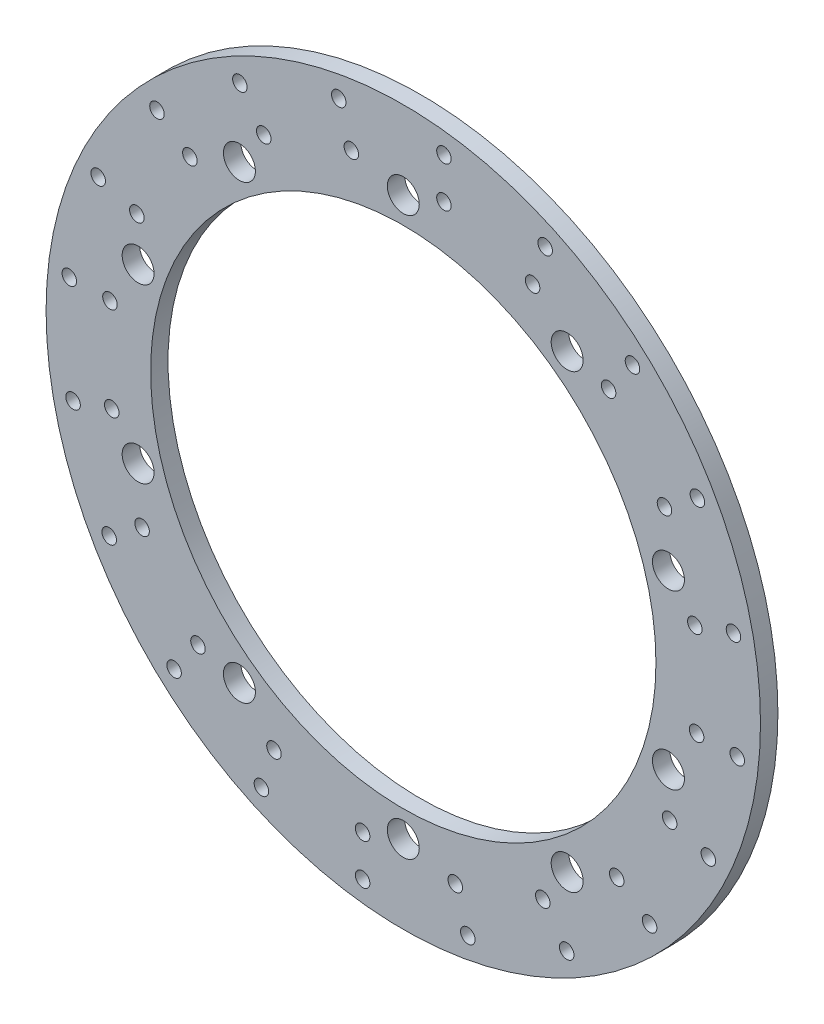
SolidWorks part; units mm, degrees
material "AL6061"
ref_plane "前视基准面" through (0, 0, 0) normal (0, 0, 1) x (1, 0, 0)
ref_plane "上视基准面" through (0, 0, 0) normal (0, 1, 0) x (1, 0, 0)
ref_plane "右视基准面" through (0, 0, 0) normal (1, 0, 0) x (0, 0, -1)
sketch "草图1" plane through (0, 0, 0) normal (0, 0, 1) x (1, 0, 0)
  circle A0 centre (0, 0) radius 61.5
  circle A1 centre (0, 0) radius 43.5
  dimension "D1" = 123
  dimension "D2" = 87
extrude "凸台-拉伸1" add sketch "草图1" along normal mid plane 3
hole_wizard "Ø5.5 (5.5) 直径孔2" positions "草图2" profile "草图3" hole size "Ø5.5" standard "GB" end condition through all
sketch "草图2" plane through (0, 0, 1.5) normal (0, 0, 1) x (1, 0, 0)
  line L0 (0, 45.7157) -> (0, -47.7003) construction
  circle A0 centre (0, 0) radius 48 construction
  point P0 (0, 48)
  dimension "D1" = 96
sketch "草图3" plane through (0, 48, 1.5) normal (1, 0, 0) x (0, -1, 0)
  line L0 (0, 0) -> (0, 3)
  line L1 (0, 3) -> (2.75, 3)
  line L2 (2.75, 3) -> (2.75, 0)
  line L5 (2.75, 0) -> (0, 0)
  line L11 (0, -6.35) -> (0, 107.95) construction
  dimension "通孔孔直径" = 5.5
  dimension "通孔孔深度" = 3
hole_wizard "M3 螺纹孔1" positions "草图4" profile "草图5" tap size "M3" standard "GB" end condition through all
sketch "草图4" plane through (0, 0, 1.5) normal (0, 0, 1) x (1, 0, 0)
  line L0 (-54, 9.4408) -> (-54, -2.1263) construction
  line L1 (5.6135, 0) -> (-69.2327, 0) construction
  point P0 (-57.5, 7)
  point P2 (-50.5, 7)
  dimension "D1" = 54
  dimension "D2" = 7
  dimension "D3" = 7
sketch "草图5" plane through (-57.5, 7, 1.5) normal (1, 0, 0) x (0, -1, 0)
  line L0 (0, 0) -> (0, 3)
  line L1 (0, 3) -> (1.25, 3)
  line L2 (1.25, 3) -> (1.25, 0)
  line L5 (1.25, 0) -> (0, 0)
  line L11 (0, -6.35) -> (0, 107.95) construction
  dimension "通孔螺纹孔钻头直径" = 2.5
  dimension "通孔螺纹孔钻头深度" = 3
cosmetic thread "孔螺蚊线1" parameters "D2"=3
cosmetic thread "孔螺蚊线2" parameters "D2"=3
pattern_circular "阵列(圆周)1" count 10 over 360 about axis through (0, 0, 0) along (0, 0, 1) of "Ø5.5 (5.5) 直径孔2"
pattern_circular "阵列(圆周)2" count 20 over 360 about axis through (0, 0, 0) along (0, 0, 1) of "M3 螺纹孔1"
